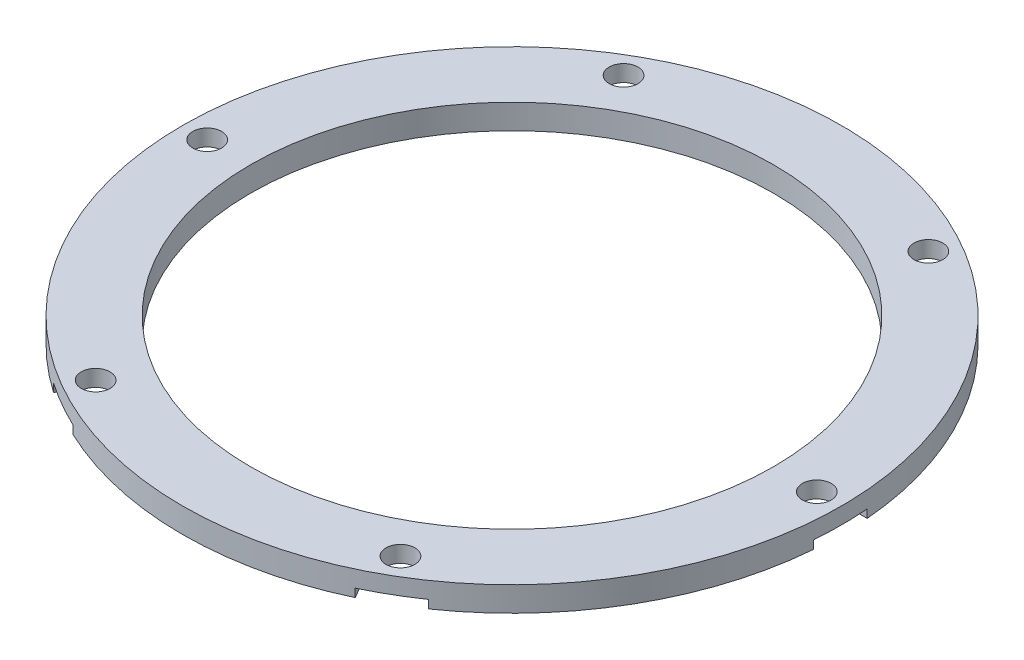
SolidWorks part; units mm, degrees
material "AISI 304"
ref_plane "Front Plane" through (0, 0, 0) normal (0, 0, 1) x (1, 0, 0)
ref_plane "Top Plane" through (0, 0, 0) normal (0, 1, 0) x (1, 0, 0)
ref_plane "Right Plane" through (0, 0, 0) normal (1, 0, 0) x (0, 0, -1)
sketch "Sketch1" plane through (0, 0, 0) normal (0, 1, 0) x (1, 0, 0)
  circle A0 centre (0, 0) radius 40
  circle A1 centre (0, 0) radius 31.75
  dimension "D1" = 63.5
  dimension "D2" = 80
extrude "Boss-Extrude1" add sketch "Sketch1" along normal blind 3
sketch "Sketch3" plane through (0, 0, 0) normal (0, -1, 0) x (1, 0, 0)
  circle A0 centre (0, 0) radius 37 construction
  circle A1 centre (37, 0) radius 1.75
  dimension "D1" = 74
  dimension "D2" = 3.5
extrude "Cut-Extrude2" cut sketch "Sketch3" against normal through all
pattern_circular "CirPattern1" count 6 over 360 about axis through (0, 0, 0) along (0, 1, 0) of "Cut-Extrude2"
sketch "Sketch5" plane through (0, 0, 0) normal (0, -1, 0) x (1, 0, 0)
  circle A0 centre (18.5, 32.0429) radius 3.25
  circle A1 centre (18.5, 32.0429) radius 1.75 construction
  dimension "D1" = 6.5
extrude "Cut-Extrude4" cut sketch "Sketch5" against normal blind 1
pattern_circular "CirPattern2" count 6 over 360 about axis through (0, 0, 0) along (0, 1, 0) of "Cut-Extrude4"
sketch "Sketch6" plane through (0, 0, 0) normal (0, -1, 0) x (1, 0, 0)
  line L0 (37, 0) -> (50037, 0) construction
  line L2 (40.5, -3.25) -> (37, -3.25)
  line L3 (40.5, -3.25) -> (40.5, 3.25)
  line L4 (40.5, 3.25) -> (37, 3.25)
  line L5 (37, -3.25) -> (37, 3.25)
  line L6 (40.5, -3.25) -> (37, 3.25) construction
  line L7 (40.5, 3.25) -> (37, -3.25) construction
  circle A0 centre (37, 0) radius 1.75 construction
  arc A1 (39.9789, 1.2995) -> (39.9789, -1.2995) centre (37, 0) ccw construction
  point P3 (38.75, 0)
extrude "Cut-Extrude5" cut sketch "Sketch6" against normal up to surface (1 mm away) up to face at (37, 1, -1.75)
pattern_circular "CirPattern3" count 6 every 60 about axis through (0, 0, 0) along (0, 1, 0) of "Cut-Extrude5"
